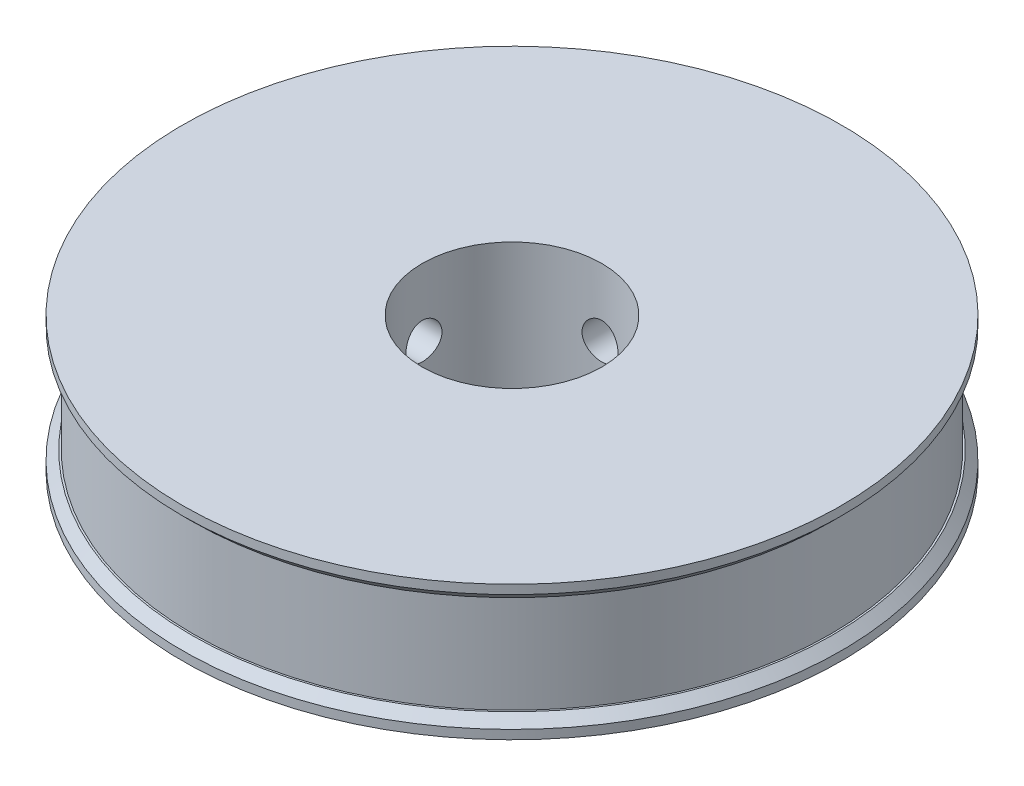
SolidWorks part; units mm, degrees
ref_plane "Front Plane" through (0, 0, 0) normal (0, 0, 1) x (1, 0, 0)
ref_plane "Top Plane" through (0, 0, 0) normal (0, 1, 0) x (1, 0, 0)
ref_plane "Right Plane" through (0, 0, 0) normal (1, 0, 0) x (0, 0, -1)
sketch "Sketch1" plane through (0, 0, 0) normal (0, 1, 0) x (1, 0, 0)
  circle A0 centre (0, 0) radius 35.5
  circle A1 centre (0, 0) radius 10
  dimension "D1" = 20
  dimension "D2" = 71
extrude "Boss-Extrude1" add sketch "Sketch1" along normal blind 11
sketch "Sketch2" plane through (0, 11, 0) normal (0, 1, 0) x (1, 0, 0)
  circle A0 centre (0, 0) radius 36.7
  circle A1 centre (0, 0) radius 35.5 construction
  circle A2 centre (0, 0) radius 10
  dimension "D1" = 1.2
  dimension "D2" = 20
extrude "Boss-Extrude2" add sketch "Sketch2" along normal blind 2
sketch "Sketch3" plane through (0, 0, 0) normal (0, -1, 0) x (1, 0, 0)
  circle A0 centre (0, 0) radius 10
  circle A1 centre (0, 0) radius 36.7
  circle A2 centre (0, 0) radius 35.5 construction
  dimension "D1" = 1.2
  dimension "D2" = 20
extrude "Boss-Extrude3" add sketch "Sketch3" along normal blind 2
chamfer "Chamfer1" distance 1 angle 45 2 edges at (0, 0, -36.7) (0, 11, 36.7)
sketch "Sketch5" plane through (0, 0, 0) normal (0, 0, 1) x (1, 0, 0)
  line L0 (0, -2.1958) -> (0, 5.5) construction
  line L1 (-10, -2) -> (10, -2) construction
  circle A0 centre (0, 5.5) radius 2
  dimension "D1" = 7.5
extrude "Cut-Extrude1" cut sketch "Sketch5" against normal blind 43
sketch "Sketch6" plane through (0, 0, 0) normal (1, 0, 0) x (0, 0, -1)
  line L0 (0, 0) -> (0, 14.0872) construction
  line L1 (-10, -2) -> (10, -2) construction
  circle A0 centre (0, 5.5) radius 2
  dimension "D1" = 7.5
extrude "Cut-Extrude2" cut sketch "Sketch6" against normal blind 43
